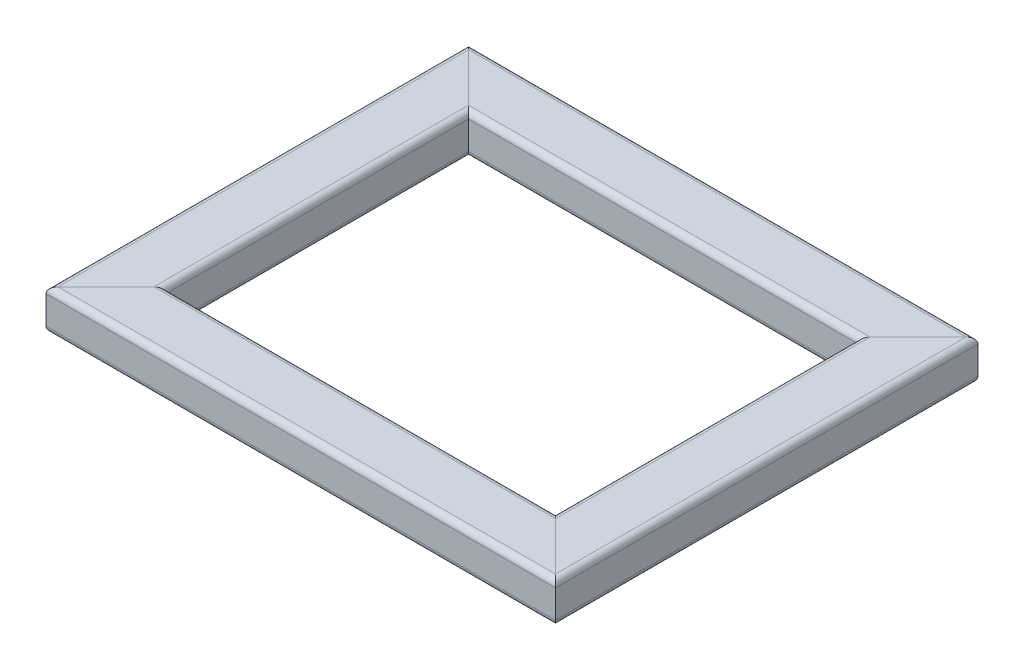
from build123d import *

# Parameters (mm, degrees)
GB_T_6728_2002_RECTANGULAR_HOLLOW_SECTIO_DEPTH      = 400.055512755
GB_T_6728_2002_RECTANGULAR_HOLLOW_SECTIO_DEPTH_BACK = 37.055512755
GB_T_6728_2002_RECTANGULAR_HOLLOW_SE_4_DEPTH        = 524.111025509
GB_T_6728_2002_RECTANGULAR_HOLLOW_SE_6_DEPTH        = 437.111025509
GB_T_6728_2002_RECTANGULAR_HOLLOW_SE_8_DEPTH        = 524.111025509


with BuildPart() as part:
    # Sketch1 → GB/T 6728-2002 Rectangular Hollow Section 60X40X3(1) (new, two sides: drawn at the far end of the back side and taken through both)
    with BuildSketch(Plane(origin=(-225, 0, 181.5), x_dir=(0, 1, 0), z_dir=(0, 0, -1)).offset(-GB_T_6728_2002_RECTANGULAR_HOLLOW_SECTIO_DEPTH_BACK)):
        with BuildLine():
            Line((-14, -30), (14, -30))
            ThreePointArc((14, -30), (18.242640687, -28.242640687), (20, -24))
            Line((20, -24), (20, 24))
            ThreePointArc((20, 24), (18.242640687, 28.242640687), (14, 30))
            Line((14, 30), (-14, 30))
            ThreePointArc((-14, 30), (-18.242640687, 28.242640687), (-20, 24))
            Line((-20, 24), (-20, -24))
            ThreePointArc((-20, -24), (-18.242640687, -28.242640687), (-14, -30))
        make_face()
        with BuildLine():
            Line((-14, -27), (14, -27))
            ThreePointArc((14, -27), (16.121320344, -26.121320344), (17, -24))
            Line((17, -24), (17, 24))
            ThreePointArc((17, 24), (16.121320344, 26.121320344), (14, 27))
            Line((14, 27), (-14, 27))
            ThreePointArc((-14, 27), (-16.121320344, 26.121320344), (-17, 24))
            Line((-17, 24), (-17, -24))
            ThreePointArc((-17, -24), (-16.121320344, -26.121320344), (-14, -27))
        make_face(mode=Mode.SUBTRACT)
    extrude(amount=GB_T_6728_2002_RECTANGULAR_HOLLOW_SECTIO_DEPTH + GB_T_6728_2002_RECTANGULAR_HOLLOW_SECTIO_DEPTH_BACK)

    # GB_T 6728-2002 Rectangular Hollow Se 2
    split(bisect_by=Plane(origin=(-225, 0, 181.5), x_dir=(0, -1, 0), z_dir=(-0.707106781, 0, -0.707106781)), keep=Keep.TOP)

    # GB_T 6728-2002 Rectangular Hollow Se 3
    split(bisect_by=Plane(origin=(-225, 0, -181.5), x_dir=(0, -1, 0), z_dir=(-0.707106781, 0, 0.707106781)), keep=Keep.TOP)


with BuildPart() as body_2:
    # Sketch1 on segment 2 (carried to segment 2) → GB_T 6728-2002 Rectangular Hollow Se 4 (new body)
    with BuildSketch(Plane(origin=(-262.055512755, 0, -181.5), x_dir=(0, 1, 0), z_dir=(1, 0, 0))):
        with BuildLine():
            Line((-14, -30), (14, -30))
            ThreePointArc((14, -30), (18.242640687, -28.242640687), (20, -24))
            Line((20, -24), (20, 24))
            ThreePointArc((20, 24), (18.242640687, 28.242640687), (14, 30))
            Line((14, 30), (-14, 30))
            ThreePointArc((-14, 30), (-18.242640687, 28.242640687), (-20, 24))
            Line((-20, 24), (-20, -24))
            ThreePointArc((-20, -24), (-18.242640687, -28.242640687), (-14, -30))
        make_face()
        with BuildLine():
            Line((-14, -27), (14, -27))
            ThreePointArc((14, -27), (16.121320344, -26.121320344), (17, -24))
            Line((17, -24), (17, 24))
            ThreePointArc((17, 24), (16.121320344, 26.121320344), (14, 27))
            Line((14, 27), (-14, 27))
            ThreePointArc((-14, 27), (-16.121320344, 26.121320344), (-17, 24))
            Line((-17, 24), (-17, -24))
            ThreePointArc((-17, -24), (-16.121320344, -26.121320344), (-14, -27))
        make_face(mode=Mode.SUBTRACT)
    extrude(amount=GB_T_6728_2002_RECTANGULAR_HOLLOW_SE_4_DEPTH)

    # GB_T 6728-2002 Rectangular Hollow Se 4 m
    split(bisect_by=Plane(origin=(225, 0, -181.5), x_dir=(0, -1, 0), z_dir=(-0.707106781, 0, -0.707106781)), keep=Keep.TOP)

    # GB_T 6728-2002 Rectangular Hollow Se 5
    split(bisect_by=Plane(origin=(-225, 0, -181.5), x_dir=(0, 1, 0), z_dir=(0.707106781, 0, -0.707106781)), keep=Keep.TOP)


with BuildPart() as body_3:
    # Sketch1 on segment 3 (carried to segment 3) → GB_T 6728-2002 Rectangular Hollow Se 6 (new body)
    with BuildSketch(Plane(origin=(225, 0, -218.555512755), x_dir=(0, 1, 0), z_dir=(0, 0, 1))):
        with BuildLine():
            Line((-14, -30), (14, -30))
            ThreePointArc((14, -30), (18.242640687, -28.242640687), (20, -24))
            Line((20, -24), (20, 24))
            ThreePointArc((20, 24), (18.242640687, 28.242640687), (14, 30))
            Line((14, 30), (-14, 30))
            ThreePointArc((-14, 30), (-18.242640687, 28.242640687), (-20, 24))
            Line((-20, 24), (-20, -24))
            ThreePointArc((-20, -24), (-18.242640687, -28.242640687), (-14, -30))
        make_face()
        with BuildLine():
            Line((-14, -27), (14, -27))
            ThreePointArc((14, -27), (16.121320344, -26.121320344), (17, -24))
            Line((17, -24), (17, 24))
            ThreePointArc((17, 24), (16.121320344, 26.121320344), (14, 27))
            Line((14, 27), (-14, 27))
            ThreePointArc((-14, 27), (-16.121320344, 26.121320344), (-17, 24))
            Line((-17, 24), (-17, -24))
            ThreePointArc((-17, -24), (-16.121320344, -26.121320344), (-14, -27))
        make_face(mode=Mode.SUBTRACT)
    extrude(amount=GB_T_6728_2002_RECTANGULAR_HOLLOW_SE_6_DEPTH)

    # GB_T 6728-2002 Rectangular Hollow Se 6 m
    split(bisect_by=Plane(origin=(225, 0, 181.5), x_dir=(0, 1, 0), z_dir=(0.707106781, 0, -0.707106781)), keep=Keep.TOP)

    # GB_T 6728-2002 Rectangular Hollow Se 7
    split(bisect_by=Plane(origin=(225, 0, -181.5), x_dir=(0, 1, 0), z_dir=(0.707106781, 0, 0.707106781)), keep=Keep.TOP)


with BuildPart() as body_4:
    # Sketch1 on segment 4 (carried to segment 4) → GB_T 6728-2002 Rectangular Hollow Se 8 (new body)
    with BuildSketch(Plane(origin=(262.055512755, 0, 181.5), x_dir=(0, 1, 0), z_dir=(-1, 0, 0))):
        with BuildLine():
            Line((-14, -30), (14, -30))
            ThreePointArc((14, -30), (18.242640687, -28.242640687), (20, -24))
            Line((20, -24), (20, 24))
            ThreePointArc((20, 24), (18.242640687, 28.242640687), (14, 30))
            Line((14, 30), (-14, 30))
            ThreePointArc((-14, 30), (-18.242640687, 28.242640687), (-20, 24))
            Line((-20, 24), (-20, -24))
            ThreePointArc((-20, -24), (-18.242640687, -28.242640687), (-14, -30))
        make_face()
        with BuildLine():
            Line((-14, -27), (14, -27))
            ThreePointArc((14, -27), (16.121320344, -26.121320344), (17, -24))
            Line((17, -24), (17, 24))
            ThreePointArc((17, 24), (16.121320344, 26.121320344), (14, 27))
            Line((14, 27), (-14, 27))
            ThreePointArc((-14, 27), (-16.121320344, 26.121320344), (-17, 24))
            Line((-17, 24), (-17, -24))
            ThreePointArc((-17, -24), (-16.121320344, -26.121320344), (-14, -27))
        make_face(mode=Mode.SUBTRACT)
    extrude(amount=GB_T_6728_2002_RECTANGULAR_HOLLOW_SE_8_DEPTH)

    # GB_T 6728-2002 Rectangular Hollow Se 8 m
    split(bisect_by=Plane(origin=(225, 0, 181.5), x_dir=(0, -1, 0), z_dir=(-0.707106781, 0, 0.707106781)), keep=Keep.TOP)

    # GB_T 6728-2002 Rectangular Hollow Se 9
    split(bisect_by=Plane(origin=(-225, 0, 181.5), x_dir=(0, 1, 0), z_dir=(0.707106781, 0, 0.707106781)), keep=Keep.TOP)


solid = Compound([part.part, body_2.part, body_3.part, body_4.part])
